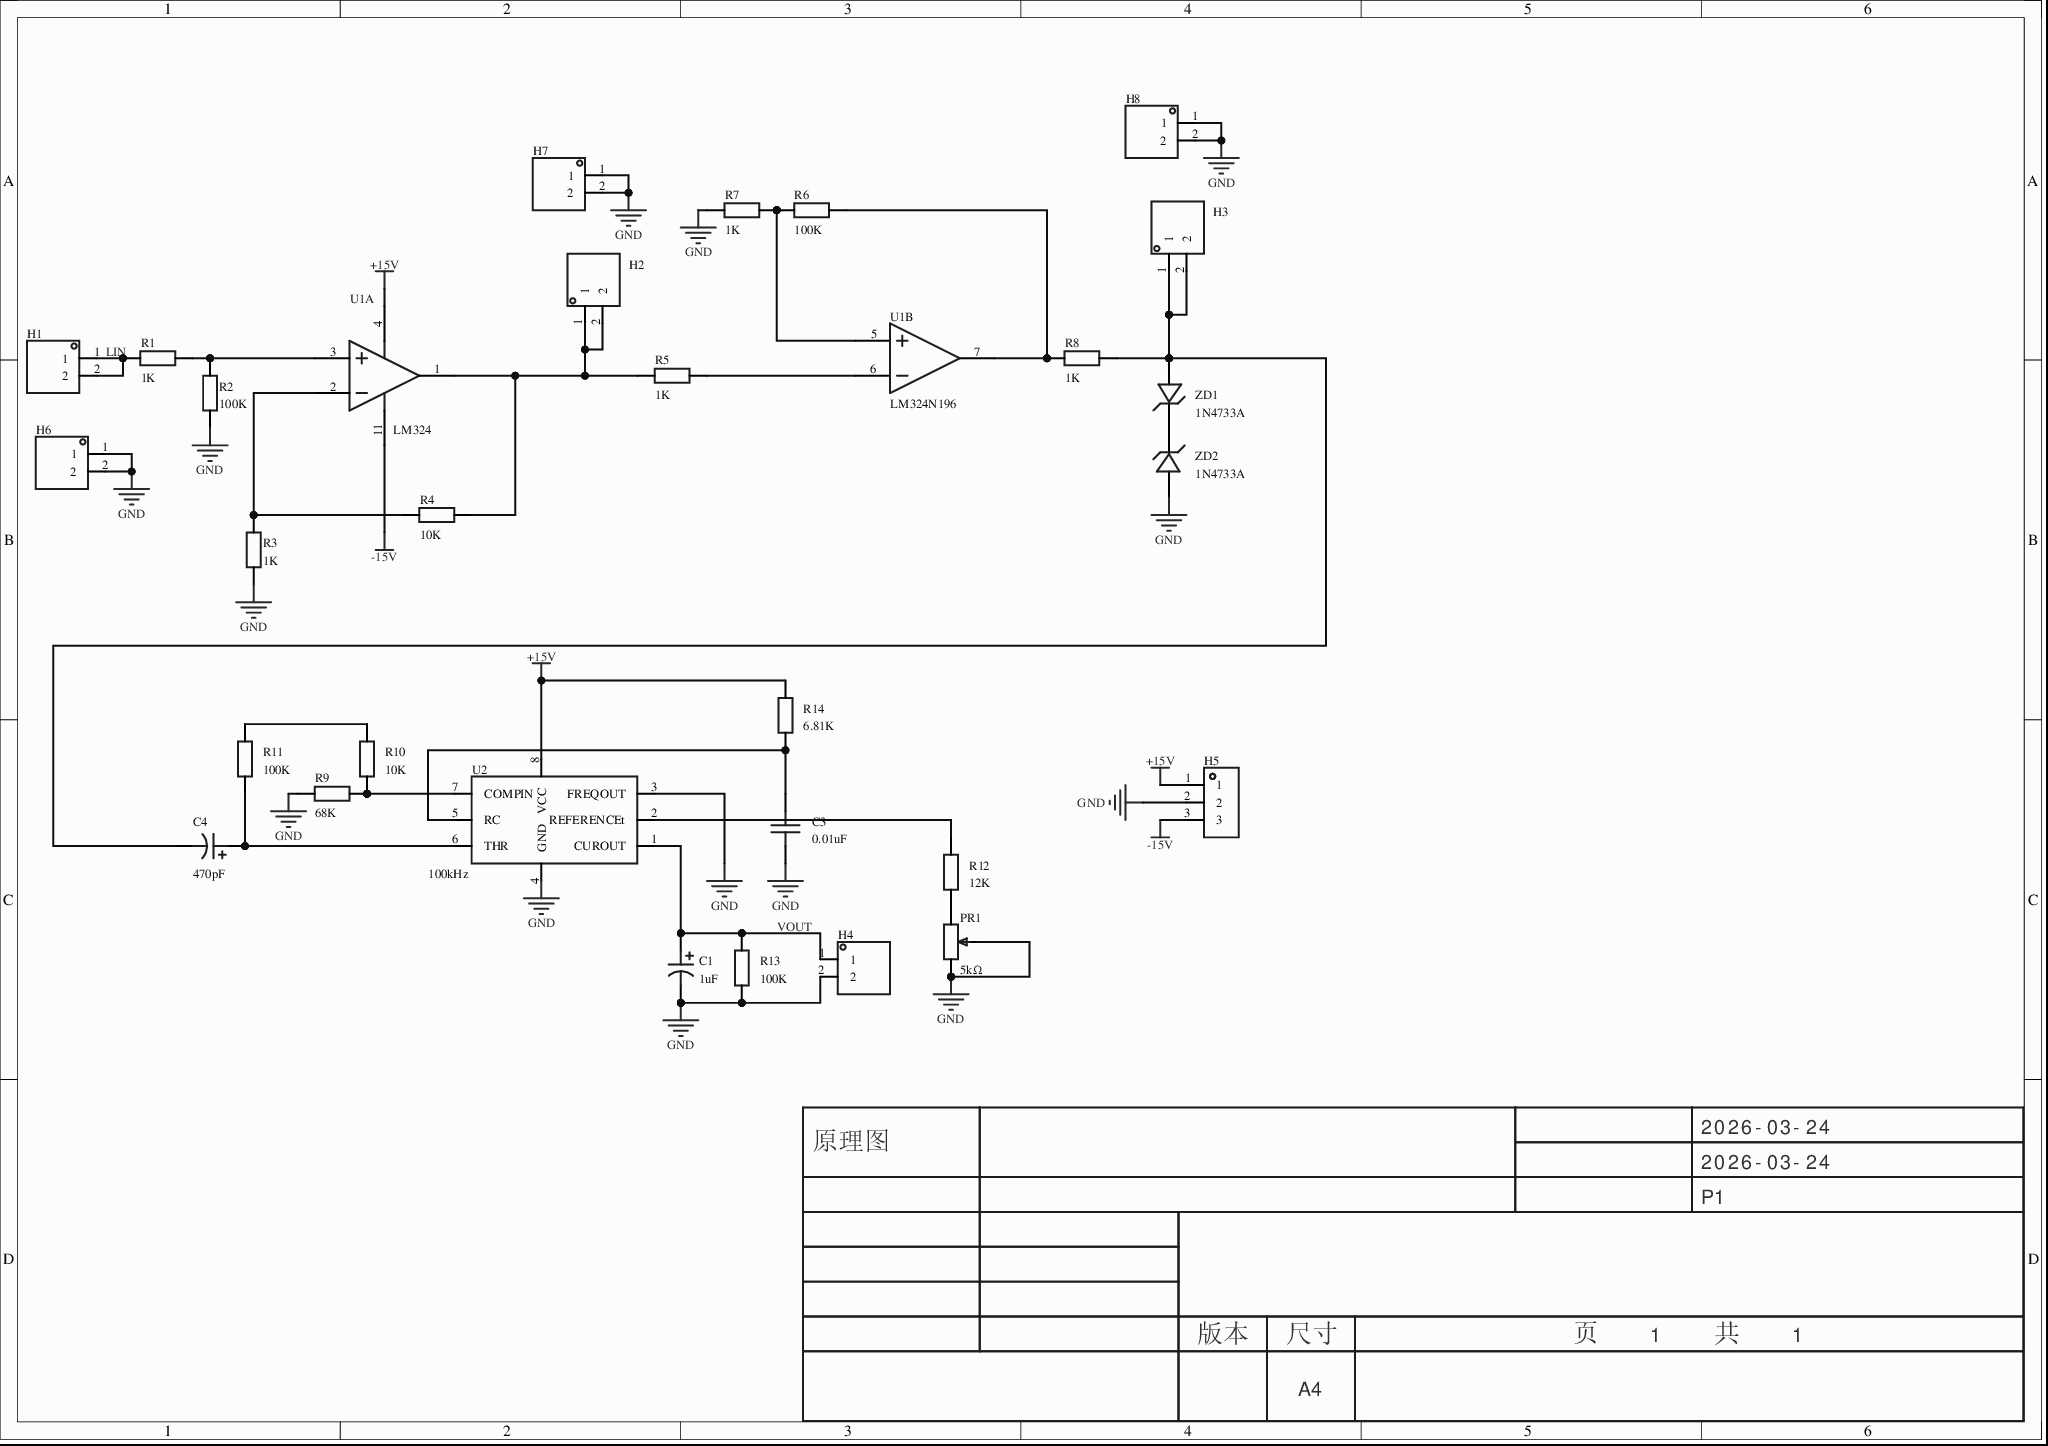
[diagram p0: MISC51973-3.schdoc]
# Altium project MISC51973-2.PrjPcb
1 sheet, 30 parts. Net scope: global (net labels, ports and power ports of the same name join across sheets).
Board file: MISC51973.pcbdoc

## Sheet MISC51973-3.schdoc
size 297 x 209 mm; Version: V1.0; @Project Name: MISC51973; @Update Date: 2026-03-24; @Create Date: 2026-03-24; @Board Name: MISC51973; @Create Time: 07:58:41; @Page Count: 1; @Page No: 1; @Schematic Name: MISC51973; @Update Time: 07:58:41; Size: A4

### Parts
C1  1uF  [CAP-TH_BD5.0-P2.00-D0.8-FD-10UF50VC110GL]
C3  0.01uF  [C0805]
C4  470pF  [CAP-TH_BD5.0-P2.00-D0.8-FD-10UF50VC110GL]
H1  (no value)  [HDR-TH_2P-P2.54-V-M-1]
H2  (no value)  [HDR-TH_2P-P2.54-V-M-1]
H3  (no value)  [HDR-TH_2P-P2.54-V-M-1]
H4  (no value)  [HDR-TH_2P-P2.54-V-M-1]
H5  (no value)  [HDR-TH_3P-P2.54-V-M]
H6  (no value)  [HDR-TH_2P-P2.54-V-M-1]
H7  (no value)  [HDR-TH_2P-P2.54-V-M-1]
H8  (no value)  [HDR-TH_2P-P2.54-V-M-1]
PR1  5kΩ  [R_3296]
R1  1K  [R0805]
R2  100K  [R0805]
R3  1K  [R0805]
R4  10K  [R0805]
R5  1K  [R0805]
R6  100K  [R0805]
R7  1K  [R0805]
R8  1K  [R0805]
R9  68K  [R0805]
R10  10K  [R0805]
R11  100K  [R0805]
R12  12K  [R0805]
R13  100K  [R0805]
R14  6.81K  [R0805]
U1  LM324  [PDIP-14_L19.3-W6.5-P2.54-LS7.6-BL]  (parts A,B of 4)
U2  100kHz  [DIP-8_L9.2-W6.4-P2.54-LS7.6-BL]
ZD1  1N4733A  [DO-41_BD2.8-L4.2-P8.00-D0.7-FD]
ZD2  1N4733A  [DO-41_BD2.8-L4.2-P8.00-D0.7-FD]

### Nets
+15V: H5.1 R14.2 U1.4(V+) U2.8(VCC)
-15V: H5.3 U1.11(V-)
GND: C1.2 C3.1 H4.2 H5.2 H6.1 H6.2 H7.1 H7.2 H8.1 H8.2 PR1.1 PR1.2 R2.1 R3.1 R7.2 R9.1 R13.1 U2.3(FREQOUT) U2.4(GND) ZD2.1(A)
LIN: H1.1 H1.2 R1.1
VOUT: C1.1 H4.1 R13.2 U2.1(CUROUT)
NetC3_2: C3.2 R14.1 U2.5(RC)
NetC4_1: C4.1 R11.1 U2.6(THR)
NetC4_2: C4.2 H3.1 H3.2 R8.1 ZD1.1(A)
NetH2_1: H2.1 H2.2 R4.2 R5.2 U1.1(OUT1)
NetPR1_3: PR1.3 R12.1
NetR1_2: R1.2 R2.2 U1.3(IN1-)
NetR3_2: R3.2 R4.1 U1.2(IN1+)
NetR5_1: R5.1 U1.6(IN2-)
NetR6_1: R6.1 R8.2 U1.7(OUT2)
NetR6_2: R6.2 R7.1 U1.5(IN2+)
NetR9_2: R9.2 R10.1 U2.7(COMPIN)
NetR10_2: R10.2 R11.2
NetR12_2: R12.2 U2.2(REFERENCEt)
NetZD1_2: ZD1.2(K) ZD2.2(K)

### Notes on the sheet
- 2026-03-24
- 原理图
- P1
- 版本
- 尺寸
- A4
- 页    1    共    1

### Library data of the parts
C1 C4 = 10UF50VC110GL: 容值:10uF;精度:±20%;额定电压:50V;纹波电流:120mA@100KHz;等效串联电阻(ESR):1.6Ω;; Manufacturer: Econd(米朗电子); AddInBom: yes; Tolerance: ±20%; Voltage Rating: 50V; Equivalent Series Resistance(ESR): 1.6Ω; Pin Spacing: 2mm; Lifetime: 5000hrs@105℃; Symbol: 10UF50VC110GL; Device: 10UF50VC110GL; LCSC Part Name: 10uF ±20% 50V; ManufacturerPart: 10UF50VC110GL; Supplier Footprint: 插件,D5xL11mm; JLCPCB Part Class: Extended Part; Datasheet: https://item.szlcsc.com/datasheet/10UF50VC110GL/49031974.html; Supplier: LCSC; ConvertToPcb: yes; FootprintName: CAP-TH_BD5.0-P2.00-D0.8-FD-10UF50VC110GL; Ripple Current: 120mA@100KHz; Diameter: 5mm; Height - Seated (Max): 11mm; Operating Temperature: -40℃~+105℃
  C1: Value: 1uF
  C4: Value: 470pF
C3 = CAP_0805: Symbol: Capacitance; ConvertToPcb: yes; ModelId: 1ba041120af144c991958decab20d2410819f05c4eef4c71ace90d822a990e87; ModelName: C0805_L2.0-W1.3-H1.3; ModelTransform: 78.74,51.181,0,0,0,0,0,0.0005,0; Device: CAP_0805; Value: 0.01uF; AddInBom: yes; Supplier Footprint: 0805; FootprintName: C0805
H1 H6-H8 = HDR-M_2.54_1x2P: Symbol: 210S-1*2P L=11.6MMGold-plated black; 3D Model: 79b2e9f2d70a4d68a1b7098f27c6d4c50819f05c4eef4c71ace90d822a990e87; 3D Model Transform: 200,100,0,0,0,0,0,0,-118.11; ConvertToPcb: yes; ModelName: HDR-M-2.54_1x2; Device: HDR-M_2.54_1x2P; Supplier Part: C124375; Supplier Footprint: 插件; AddInBom: yes; FootprintName: HDR-TH_2P-P2.54-V-M-1
H2-H4 = HDR-M_2.54_1x2P: Symbol: 210S-1*2P L=11.6MMGold-plated black; ConvertToPcb: yes; ModelId: 79b2e9f2d70a4d68a1b7098f27c6d4c50819f05c4eef4c71ace90d822a990e87; ModelName: HDR-M-2.54_1x2; ModelTransform: 200,100,0,0,0,0,0,0,-118.11; Device: HDR-M_2.54_1x2P; AddInBom: yes; SupplierPart: C124375; Supplier Footprint: 插件; FootprintName: HDR-TH_2P-P2.54-V-M-1
H5 = HDR-M_2.54_1x3P: AddInBom: yes; ModelId: bb473b6d38ff42a99216a4fcdbdcc4cb0819f05c4eef4c71ace90d822a990e87; ModelName: HDR-TH_3P-P2.54-M-LI-1X3P; ModelTransform: 300.03877,100,0,0,0,0,0,0,-118.11; Symbol: HDR-M_2.54_1x3P; Device: HDR-M_2.54_1x3P; ConvertToPcb: yes; FootprintName: HDR-TH_3P-P2.54-V-M; SupplierPart: C2937625; Supplier Footprint: 插件
PR1 = R_3296: ConvertToPcb: yes; ModelId: b182808559bb43bda9e7de64b64134cb0819f05c4eef4c71ace90d822a990e87; ModelName: 3296W; ModelTransform: 373.98,188.96,590.49,180,0,0,0,0,-140; Symbol: R_3296; Device: R_3296; Value: 5kΩ; AddInBom: yes; Supplier Footprint: 直插; FootprintName: R_3296
R1-R14 = Res_0805: Symbol: 电阻; ConvertToPcb: yes; ModelId: 37a81e68749a4138bd2dfa6897b24b850819f05c4eef4c71ace90d822a990e87; ModelName: R0805_L2.0-W1.3-H0.6; ModelTransform: 78.74,51.181,0,0,0,0,0,-0.0005,0; Device: Res_0805; AddInBom: yes; Supplier Footprint: 0805; FootprintName: R0805
  R1 R3 R5 R7 R8: Value: 1K
  R2 R6 R11 R13: Value: 100K
  R4 R10: Value: 10K
  R9: Value: 68K
  R12: Value: 12K
  R14: Value: 6.81K
U1 = LM324N196: 放大器数:4;轨到轨:-;增益带宽积(GBW):-;输入失调电压(Vos):2mV;压摆率(SR):400V/ms;输入偏置电流(Ib):250nA;; Manufacturer: GMIC(绿微); Relevance: []; AddInBom: yes; ModelId: 7604059b31ae49f98a0332a7cce2343e0819f05c4eef4c71ace90d822a990e87; ModelTransform: 759.15391,311.417,0,0,0,0,0,0,-129.921; Number of Channels: 4; Maximum Power Supply Range (Vdd-Vss): 24V; Vos - Input Offset Voltage: 2mV; Input Offset Voltage Drift(Vos TC): 7uV/℃; Ib - Input Bias Current: 250nA; Input Offset Current(Ios): 5nA; Common Mode Rejection Ratio(CMRR): 80dB; Quiescent Current: 600uA; Output Current: 40mA; Single supply: 3V~24V; Dual Supply: -12V~-1.5V；1.5V~12V; Symbol: LM324N196; Device: LM324N196; Manufacturer Part: LM324; LCSC Part Name: 高性能四独立运算放大器; SupplierPart: C51026325; Supplier Footprint: DIP-14; JLCPCB Part Class: Extended Part; Datasheet: https://item.szlcsc.com/datasheet/LM324N196/53673003.html; Supplier: LCSC; ConvertToPcb: yes; FootprintName: PDIP-14_L19.3-W6.5-P2.54-LS7.6-BL; ModelName: PDIP-14_L19.3-W6.5-P2.54-LS7.6-BL; Rail to Rail: -; Gain Bandwidth Product: -; Slew Rate: 400V/ms; Input offset current drift(Ios TC): -; Operating Temperature: 0℃~+70℃
U2 = LM331: 工作电压:40V;频率:100kHz;转换类型VF/FV:V/F;; Manufacturer: Slkor(萨科微); AddInBom: yes; ModelId: 0f67547f9f69422e93d8ef5b6ef310c70819f05c4eef4c71ace90d822a990e87; ModelTransform: 358.267,309.999,0,0,0,0,-0.004,0.002,-125.984; Voltage - Supply: 40V; Linearity: 0.01%; Conversion Type VF/FV: V/F; Temperature Stability: 60ppm/℃; Pd - Power Dissipation: 500mW; Vos - Input Offset Voltage: 10mV; Ib - Input Bias Current: 80nA; Input Offset Current(Ios): 8nA; Symbol: LM331; Device: LM331; LCSC Part Name: 电压频率转化器; SupplierPart: C3041283; ManufacturerPart: LM331; Supplier Footprint: DIP-8; JLCPCB Part Class: Extended Part; Datasheet: https://item.szlcsc.com/datasheet/LM331/3601242.html; Supplier: LCSC; ConvertToPcb: yes; FootprintName: DIP-8_L9.2-W6.4-P2.54-LS7.6-BL; ModelName: DIP-8_L9.2-W6.4-P2.54-LS7.6-BL; Value: 100kHz; Operating Temperature: 0℃~+70℃
ZD1 ZD2 = 1N4733A: 二极管配置:独立式;稳压值(标称值):5.1V;稳压值(范围):4.84V~5.36V;耗散功率(Pd):1W;; Manufacturer: ST(先科); Symbol: 1N4733A_C2536; AddInBom: yes; ModelId: 60a9ba1ea4e145a09c5109b7504cfdbe0819f05c4eef4c71ace90d822a990e87; ModelName: DO-41_D2.8-L4.2-P8.00; ModelTransform: 346.456,102.309,0,180,0,0,0,0,-137.795; Diode Configuration: 独立式; Zener Voltage(Nom): 5.1V; Reverse Leakage Current (Ir): 10uA@1V; Pd - Power Dissipation: 1W; Impedance(Zzt): 7Ω; Impedance(Zzk): 550Ω; Device: 1N4733A; LCSC Part Name: 停产 1N4733A; SupplierPart: C2536; ManufacturerPart: 1N4733A; Supplier Footprint: DO-41; JLCPCB Part Class: Extended Part; Datasheet: https://item.szlcsc.com/datasheet/1N4733A/2913.html; Supplier: LCSC; ConvertToPcb: yes; FootprintName: DO-41_BD2.8-L4.2-P8.00-D0.7-FD; Zener Voltage(Range): 4.84V~5.36V